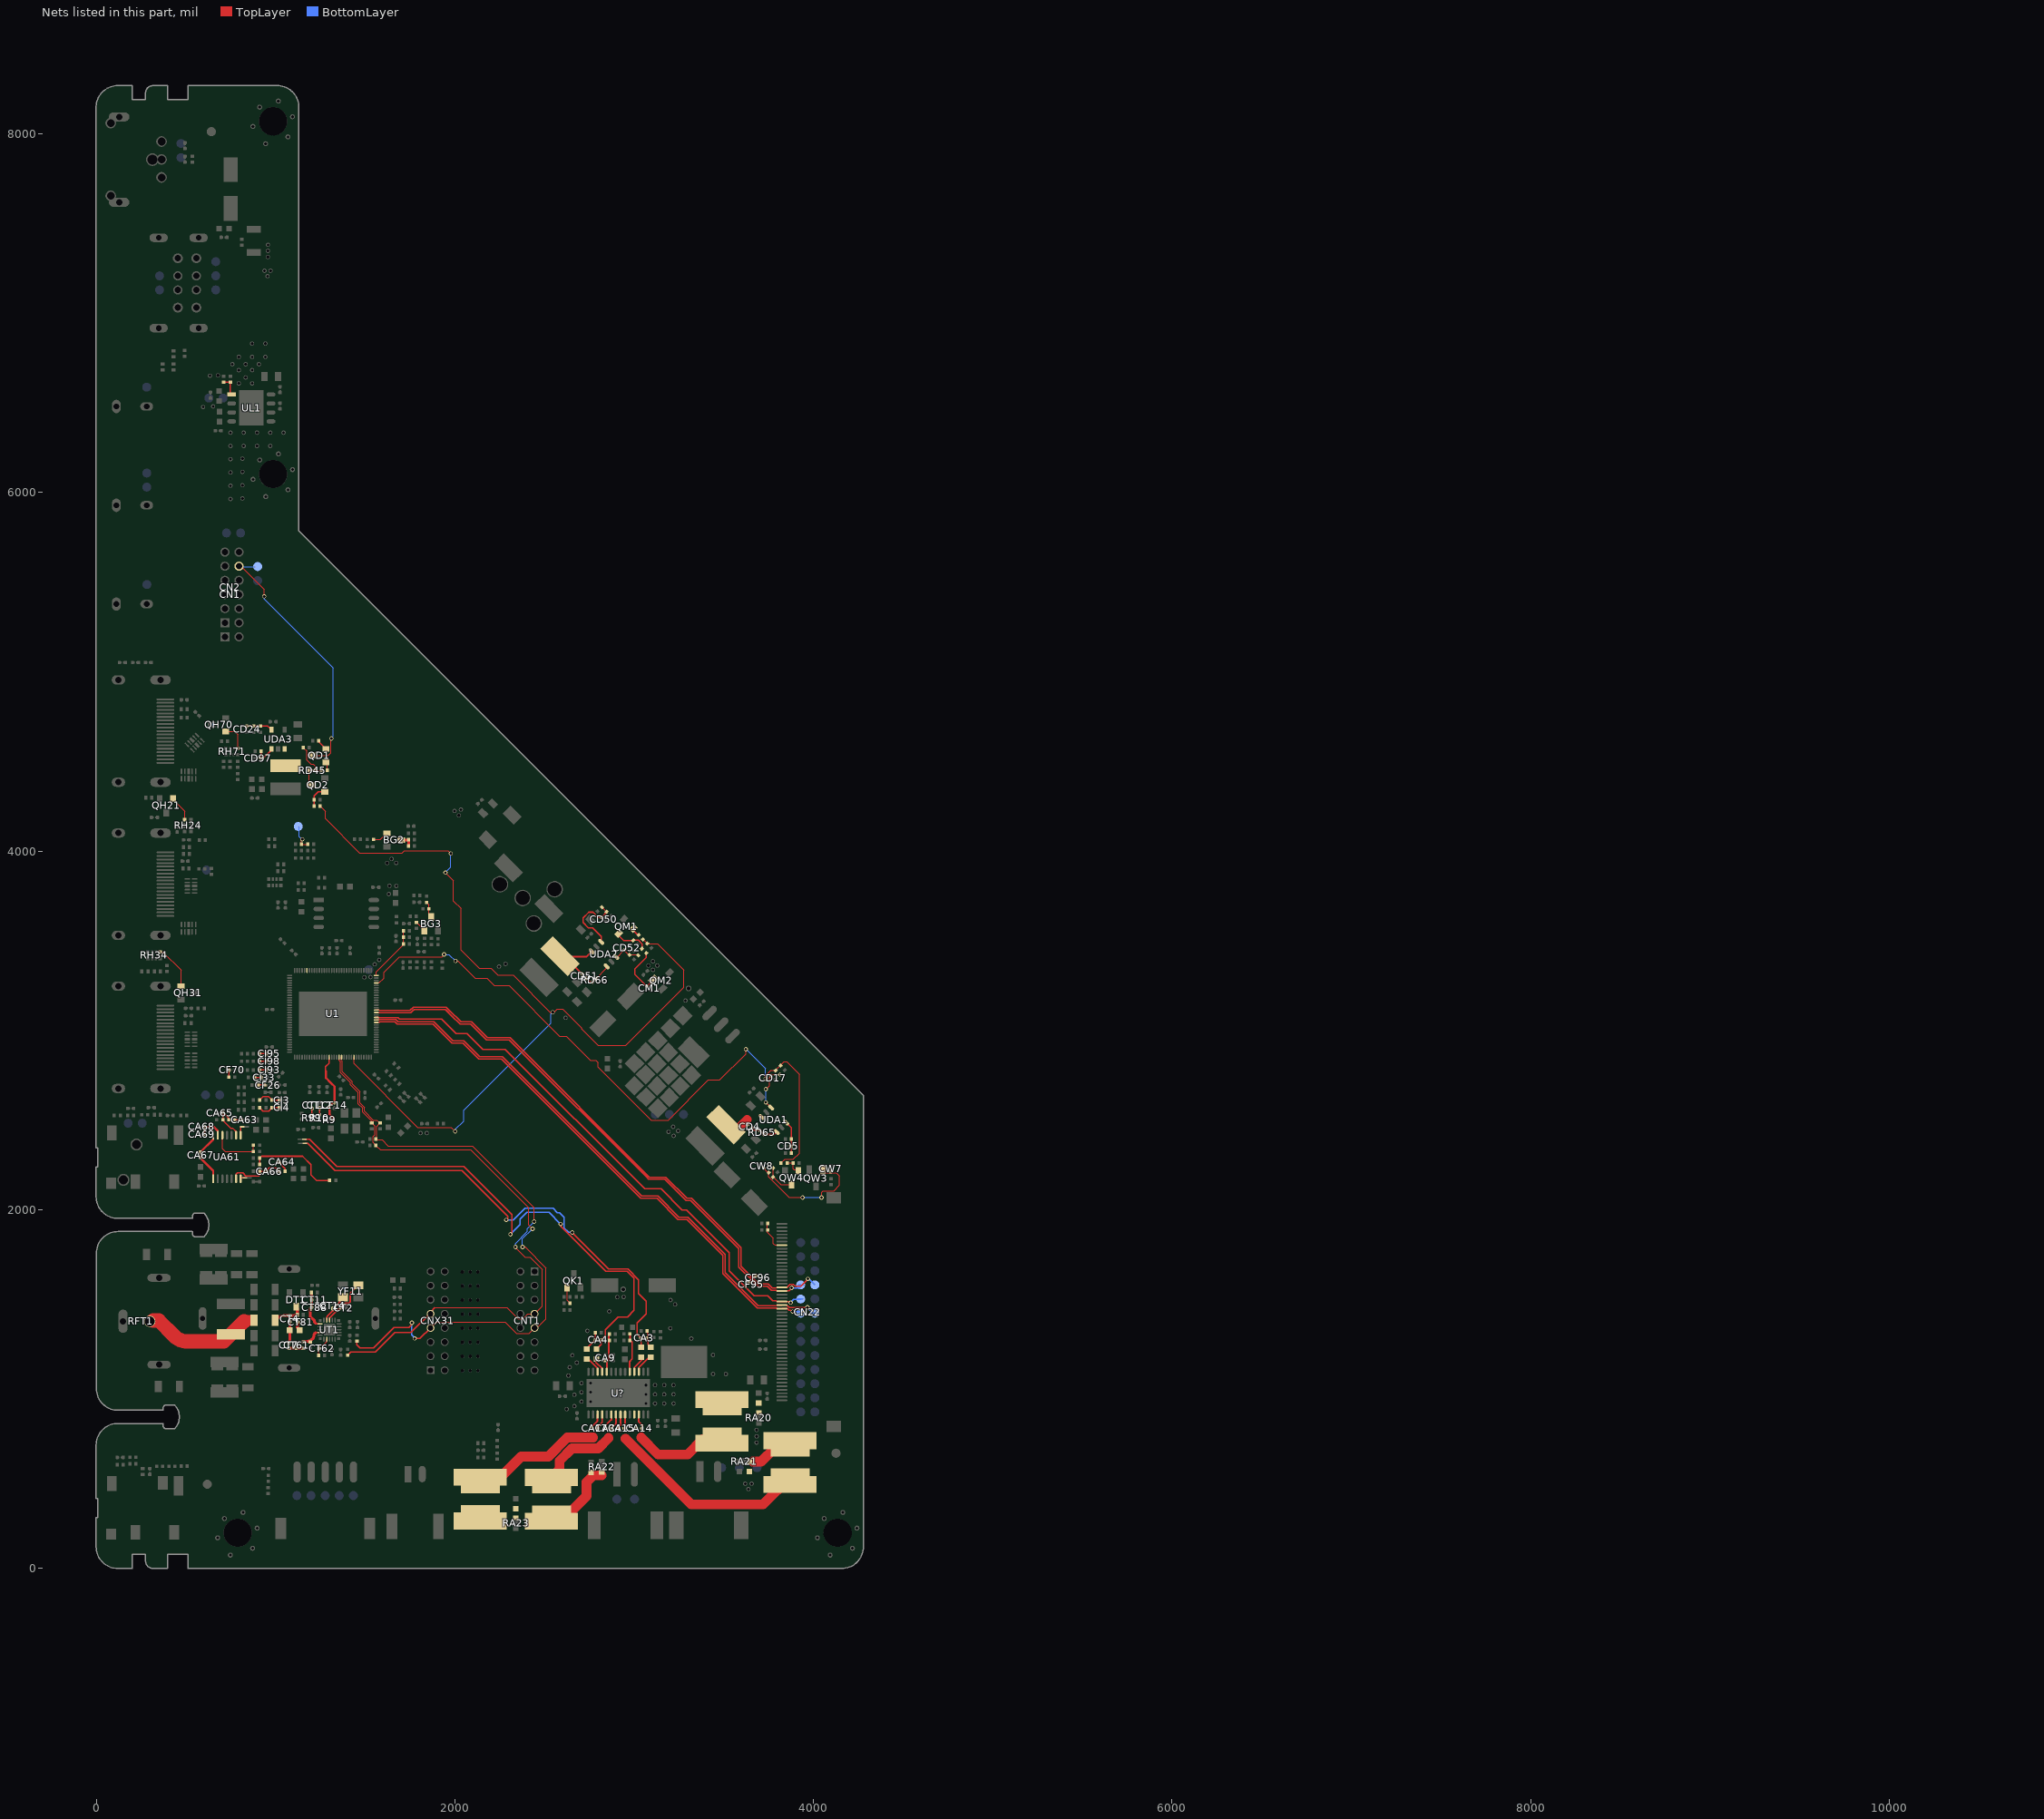
[diagram p0: the nets of this part, all layers, seen from the top]
# Altium PCB MISC105950.PcbDoc (part 12 of 15)
Units mil, origin at the board's own origin, x right, y up, seen from the top; angles counter-clockwise.
Board outline 4280.62 x 8272.76 mil, 2 copper layers (TopLayer, BottomLayer), stack 61.855 mil thick; 541 components, 268 nets, 2324 pads, 1157 vias.

## Via types
v1: diameter 23.62, hole 15.75, TopLayer to BottomLayer, tented both sides, 1087 vias
v2: diameter 23.62, hole 15.75, TopLayer to BottomLayer, 51 vias
v3: diameter 27.56, hole 19.68, TopLayer to BottomLayer, 15 vias
v4: diameter 31.5, hole 19.68, TopLayer to BottomLayer, tented both sides, 4 vias

## Nets (pads, with @x,y where several pads share a name; then routed paths per layer and width w, separated by ;. In a path a pad name is that pad's centre, name@x,y a point inside that pad or via, vN(x,y) a via of type N, cw(c..) or ccw(c..) an arc to the next point about the centre after c; other vN are vias at no path point) (continued)
LVDS_O3P_IC: CN22.29 O3P.1 U1.79 | length 3126.4
  TopLayer w7: U1.79@1560.66,3071.21 1561.61,3072.16 1573.58,3072.16 1574.53,3071.21 1682.5,3071.21 1690.21,3063.5 1924.1,3063.5 2005.42,2982.18 2066.04,2982.18 2154.53,2893.69 2279.87,2893.69 3058.06,2115.5 3148.94,2115.5 3266.39,1998.05 3291.64,1998.05 3529.95,1759.73 3529.95,1657.23 3668.17,1519.01 3744.26,1519.01 3773.37,1489.9 3791.5,1489.9 3794.99,1486.41 CN22.29@3823.43,1486.41 3866.09,1486.41 v1(3872,1480.5)
  BottomLayer w7: v1@3872,1481.5 3888.5,1498 3925.82,1498 O3P.1@3928.5,1500.68 ; O3P.1@3910.18,1500.68 O3P.1@3928.5,1500.68 ; O3P.1@3941.07,1500.68 O3P.1@3928.5,1500.68
LVDS_O4N_IC: CN22.28 O4N.1 U1.78 | length 3165.9
  TopLayer w7: U1.78@1560.66,3057.43 1574.47,3057.43 1576.25,3059.21 1669.47,3059.21 1681.18,3047.5 1882.12,3047.5 1988.44,2941.18 2049.06,2941.18 2137.55,2852.69 2262.89,2852.69 3041.07,2074.5 3131.95,2074.5 3249.41,1957.05 3298.7,1957.05 3505.95,1749.79 3505.95,1647.28 3690.71,1462.53 3790,1462.53 3794.19,1466.72 CN22.28@3823.43,1466.72 ; CN22.28@3851.75,1466.72 3866.24,1452.24 3964.24,1452.24 v1(3966,1454)
  BottomLayer w7: v1(3966,1454) 3966,1450 3994.06,1421.94 O4N.1@4007.24,1421.94 ; O4N.1@4006.68,1421.38 O4N.1@4007.24,1421.94 ; O4N.1@4007.24,1421.3 O4N.1@4007.24,1421.94
LVDS_O4P_IC: CN22.27 O4P.1 U1.77 | length 3079
  TopLayer w7: U1.77@1560.66,3043.65 1561.61,3044.6 1578.61,3044.6 1581.22,3047.21 1664.5,3047.21 1676.21,3035.5 1877.15,3035.5 1983.47,2929.18 2044.09,2929.18 2132.58,2840.69 2257.92,2840.69 3036.1,2062.5 3126.98,2062.5 3244.44,1945.05 3293.73,1945.05 3493.95,1744.82 3493.95,1642.31 3685.74,1450.53 3791.5,1450.53 CN22.27@3794.99,1447.04 ; CN22.27@3823.43,1447.04 3854.46,1447.04 3862.5,1439 v1@3875,1439
  BottomLayer w7: v1(3883,1431) 3919.44,1431 O4P.1@3928.5,1421.94 ; O4P.1@3925.94,1424.5 O4P.1@3928.5,1421.94 ; O4P.1@3941.03,1421.94 O4P.1@3928.5,1421.94
LVDS_OCKN_IC: CF96.2@3676.78,1631.31 CF96.2@3681.65,1626.44 CN22.33 OCKN.1 U1.82 | length 3312.3
  TopLayer w7: U1.82@1560.66,3112.55 1576.22,3112.55 ; 1578,3110.77 1745.38,3110.77 1745.19,3110.96 1748.67,3110.96 ; 1762.22,3124.5 1748.67,3110.96 ; 1955.03,3124.5 1967.93,3111.59 ; 3594.95,1762.61 3594.95,1714 ; CF96.2@3676.49,1631.31 CF96.2@3676.78,1631.31 3663.67,1618.2 3660.9,1618.2 ; v1@3966,1610 3928,1572 3897.72,1572 3886.41,1583.31 3884,1583.31 3869.59,1583.31 3851.42,1565.15 CN22.33@3823.43,1565.15 3794.19,1565.15 3790,1560.95 3770.2,1560.95 3747.15,1584.01 3695.1,1584.01 3660.9,1618.2 ; 1748.67,3110.96 1766.72,3129 1950.53,3129 1967.93,3111.59 ; 1967.93,3111.59 2032.35,3047.18 2092.97,3047.18 2115.07,3025.07 2181.45,2958.69 2306.79,2958.69 3084.98,2180.5 3175.86,2180.5 3293.31,2063.05 3318.56,2063.05 3594.95,1786.65 3594.95,1714 ; 3594.95,1714 3594.95,1684.15 3660.9,1618.2
  BottomLayer w7: v1@3966,1610 3976.66,1610 OCKN.1@4007.24,1579.42
  other v1: 3968,1613
LVDS_OCKP_IC: CF95.2@3639.03,1593.85 CF95.2@3643.9,1588.98 CN22.32 OCKP.1 U1.81 | length 3215.3
  TopLayer w7: U1.81@1560.66,3098.77 1753.45,3098.77 1760.09,3105.41 ; 1767.19,3112.5 1760.09,3105.41 ; 1950.06,3112.5 1981.19,3081.37 ; CF95.2@3639.03,1593.85 3651.63,1606.45 ; v1(3878,1563) 3878,1559 3864.46,1545.46 CN22.32@3823.43,1545.46 3794.99,1545.46 3791.5,1548.95 3765.23,1548.95 3742.18,1572.01 3690.13,1572.01 3582.95,1679.18 3582.95,1781.68 3313.59,2051.05 3288.34,2051.05 3170.89,2168.5 3080.01,2168.5 3070.26,2178.26 2301.82,2946.69 2176.48,2946.69 2087.99,3035.18 2027.38,3035.18 1981.19,3081.37 ; 1760.09,3105.41 1771.69,3117 1945.56,3117 1981.19,3081.37
  BottomLayer w7: v1(3878,1563) 3920.58,1563 OCKP.1@3937,1579.42 ; OCKP.1@3914.42,1579.42 OCKP.1@3928.5,1579.42 OCKP.1@3937,1579.42 ; OCKP.1@3946.58,1579.42 OCKP.1@3937,1579.42
LVDS_SEL: CN22.45 RF4.1 RF5.2 | length 176.6
  TopLayer w5: RF4.1@3741.71,1920.77 3741.71,1873.24 3775.5,1839.45 3775.5,1809.5 3783.63,1801.37 CN22.45@3823.43,1801.37
MAIN_SCL_OUT_IC: CNT1.7 CNX31.9 DK3.K RF43.2 RT2.1 U1.52 | length 3560.2
  TopLayer w5: U1.52@1366.73,2849.72 1366.73,2832.27 1369.84,2829.16 1369.84,2768.82 1425.8,2712.86 1425.8,2701.79 1469.66,2657.93 1469.66,2593.48 1493.5,2569.64 1493.5,2547.85 1542.26,2499.09 1564.05,2499.09 1580.41,2482.73 DK3.K@1581.5,2482.73 1562.83,2464.06 1562.83,2397.36 RF43.2@1558.96,2393.5 1564.15,2388.31 1594,2388.31 1627.31,2355 2095.83,2355 2441,2009.83 2441,1961.5 ; 1888,1452 2289.13,1452 2352.4,1388.74 2376.55,1388.74 2405.7,1417.89 CNT1.7@2443.21,1417.89 2485.5,1460.18 2485.5,1665.73 2417.05,1734.19 2390,1734.19 v1@2336.5,1787.69 ; v1@2441,1931.5 2441,1961.5 ; v1(2441,1932.5) 2441,1961.5
  TopLayer w7: RT2.1@1401,1187.77 1417.73,1204.5 1555.94,1204.5 1664.44,1313 1753.89,1313 1858.84,1417.95 CNX31.9@1863.21,1417.95 1863.21,1427.21 1888,1452
  BottomLayer w5: v1(2336.5,1791) 2336.5,1810.64 2403,1877.14 2403,1893.5 v1@2441,1931.5
MAIN_SDA_IO_IC: CNT1.9 CNX31.7 DK2.K RF44.2 RT3.1 U1.51 | length 3623.1
  TopLayer w5: U1.51@1351.85,2848.62 U1.51@1352.95,2849.72 1352.95,2831.91 1359.84,2825.02 1359.84,2764.68 1416.7,2707.82 1416.7,2696.75 1459.66,2653.79 1459.66,2589.34 1483.5,2565.5 1483.5,2543.71 1534.5,2492.71 DK2.K@1534.5,2482.73 1552.83,2464.41 1552.83,2416.67 1542.61,2406.45 1542.61,2373.86 RF44.2@1558.96,2357.5 1582.46,2334 2087.13,2334 2410.5,2010.63 2410.5,1913.96 v1@2431.96,1892.5 ; CNX31.7@1863.21,1339.21 1897,1373 2280,1373 2343,1310 2414.06,1310 CNT1.9@2443.21,1339.15 2455.15,1339.15 2506.5,1390.5 2506.5,1674.43 2389.93,1791 v1(2376.5,1791)
  TopLayer w7: RT3.1@1452,1265.27 1452,1245 1468.5,1228.5 1546,1228.5 1658,1340.5 1742.5,1340.5 1758.81,1356.81 v1(1758.81,1368.56) ; v1(1775,1280.5) 1804.5,1280.5 CNX31.7@1863.21,1339.21
  BottomLayer w5: v1(2376.5,1791) 2376.5,1836.5 v1(2432.5,1892.5)
  BottomLayer w7: v1@1761.31,1366.06 v1(1758.81,1368.56) 1758.81,1299.95 1775,1283.77 v1(1775,1280.5)
MHL_5V_IN_IC: U1.123
NetBG2_B: BG2.B RG1.1 | length 83.8
  TopLayer w5: RG1.1@1544.23,4064.5 1583.5,4064.5 BG2.B@1615,4096
NetBG2_C: BG2.C RG6.2 RG66.1 | length 84.6
  TopLayer w5: BG2.C@1693.03,4058 BG2.C@1698.53,4058
  TopLayer w15: BG2.C@1698.53,4061 1738.02,4061 1740.77,4063.75 RG66.1@1740.77,4028
NetBG3_B: BG3.B RG2.1 | length 64.1
  TopLayer w5: RG2.1@1784.5,3601.73 1826.5,3559.73 BG3.B@1826.5,3555
NetBG3_C: BG3.C RG7.2 RG67.1 | length 91.5
  TopLayer w5: RG7.2@1841,3713.77 1854.73,3700.04 RG67.1@1854.73,3677.5 1854.73,3645.3 BG3.C@1867,3633.03
NetCA3_1: CA3.1 CA6.1 RA4.JP_1K | length 2721.9
  TopLayer w7: RA4.JP_1K@1162,2368.34 1179.08,2368.34 1330.42,2217 2038.66,2217 2293.5,1962.16 v1@2293.5,1942 ; v1@2653,1871.5 2856,1668.5 2963.78,1668.5 3024,1608.28 3024,1530.59 3066.95,1487.63 3066.95,1417.74 3015.13,1365.91 3015.13,1303.64 CA3.1@3036.27,1282.5 3038,1280.77 CA6.1@3038,1231.81 ; CA6.1@3041.77,1226.04 CA6.1@3041.77,1231.81
  BottomLayer w7: v1@2285,1938.51 v1(2285,1942) 2324.82,1942 2390.13,2007.31 2546.16,2007.31 2570.97,1982.5 2584,1982.5 2609.31,1957.19 2609.31,1907 2609.31,1895.94 2633.25,1872 v1(2653.5,1872)
NetCA3_2: CA3.2@3062.85,1282.5 CA3.2@3069.74,1282.5 CA5.1 RA3.2 | length 102.4
  TopLayer w7: 3072.5,1310.5 3072.5,1272.73 3075.23,1270 3075.23,1247.08 CA5.1@3102,1220.31
NetCA4_1: CA4.1 CA11.1 RA14.2 | length 107.6
  TopLayer w7: CA11.1@2739.5,1222.31 2739.5,1230.44 CA4.1@2782.3,1273.23 RA14.2@2782.29,1312.23
NetCA4_2: CA4.2@2808.87,1273.23 CA4.2@2815.76,1273.23 CA10.1 RA5.JP_1K | length 2861.6
  TopLayer w7: RA5.JP_1K@1160,2392.34 1189.02,2392.34 1340.37,2241 2048.61,2241 2317.5,1972.11 2317.5,1870.5 v1(2309,1862) ; 2589,1907.3 2839.8,1656.5 2958.81,1656.5 2998,1617.31 2998,1437 2961.5,1400.5 2908.5,1400.5 2837.5,1329.5 2837.5,1294.97 CA4.2@2815.76,1273.23 2815.76,1248.14 CA10.1@2788.94,1221.32
  BottomLayer w7: v1(2309,1862) 2363,1916 2363,1946.24 2400.07,1983.31 2524.47,1983.31 v1@2588.28,1919.5
  other v1: 2589,1919.5
NetCA5_2: CA5.2 U?.3 | length 114.2
  TopLayer w7: U?.3@3025.36,1094.5 3025.36,1117.86 3083.69,1176.19 CA5.2@3092,1176.19
NetCA6_2: CA6.2 U?.4 | length 164.3
  TopLayer w7: U?.4@2999.77,1094.5 2999.77,1118.77 ; CA6.2@3038,1176.19 3038,1157 2999.77,1118.77 ; CA6.2@3047.5,1164.69 3045.69,1164.69 2999.77,1118.77
NetCA9_2: CA9.2@2837.44,1155.77 CA9.2@2837.44,1162.66 RA10.2 RA11.2 U?.10 | length 219.3
  TopLayer w10: CA9.2@2837.44,1155.77 2847.7,1155.77 2858.07,1166.13 2858.07,1303.37 RA11.2@2860.21,1305.5 ; U?.10@2846.23,1094.5 2846.23,1146.98 ; RA10.2@2858.07,1262.37 RA10.2@2859.21,1263.5
NetCA10_2: CA10.2 U?.11 | length 86.3
  TopLayer w7: CA10.2@2786.5,1166.69 2786.5,1147.5 2820.64,1113.36 U?.11@2820.64,1094.5
NetCA11_2: CA11.2 U?.12 | length 93.8
  TopLayer w7: CA11.2@2742.98,1166.69 2795.05,1114.62 U?.12@2795.05,1094.5
NetCA14_1: CA14.1 U?.26 | length 76.9
  TopLayer w10: U?.26@3025.36,854.34 3025.36,825.78 3025.5,825.64 3025.5,815.23 3043.73,797 CA14.1@3043.73,785
NetCA14_2: CA14.2@3010.26,779 CA14.2@3017.15,779 LA1.2 LA5.S U?.25 | length 417.8
  TopLayer w55: 3038,727.5 3132.33,633.17 3297.55,633.17 LA1.2@3381.83,717.45
NetCA15_1: CA15.1 U?.22 | length 79.8
  TopLayer w10: CA15.1@2912.27,779 2912.27,786.68 2923,797.41 U?.22@2923,854.34
NetCA15_2: CA15.2@2938.85,779 CA15.2@2945.74,779 LA2.F LA3.1 U?.23 | length 1208.6
  TopLayer w10: CA15.2@2945.74,779 2948.59,781.85 U?.23@2948.59,854.34
  TopLayer w55: 2951.25,721.75 3318,355 3718.37,355 LA2.F@3869,505.63
NetCA17_1: CA17.1 U?.17 | length 88.1
  TopLayer w10: CA17.1@2764.27,779 2764.27,789.32 2795.05,820.09 U?.17@2795.05,854.34
NetCA17_2: CA17.2@2790.85,779 CA17.2@2797.74,779 LA4.F LA8.1 U?.18 | length 845.4
  TopLayer w10: CA17.2@2797.74,779 2797.74,789.74 2820.64,812.64 U?.18@2820.64,854.34
  TopLayer w55: LA4.F@2140.5,466.87 LA8.1@2140.5,506.05 2253.05,506.05 2369.32,622.32 2520.86,622.32 2625.79,727.25 2770.25,727.25
NetCA20_2: CA20.2 LA1.1 LA5.F RA20.1
NetCA21_1: CA21.1 LA2.S LA3.2 RA21.1 | length 239.9
  TopLayer w55: 3661.14,594 3708.5,594 3785.87,671.37 LA2.S@3869,671.37
NetCA22_2: CA22.2 LA6.2 LA7.S RA22.1 | length 415.2
  TopLayer w55: LA7.S@2538,300.17 2632.67,300.17 2733.5,401 2733.5,479 2770.86,516.36 2818,516.36
NetCA23_1: CA23.1 LA4.S LA8.2 RA23.1
NetCA34_1: CA34.1 U?.21 | length 85.8
  TopLayer w10: CA34.1@2872.23,779 2897.41,804.18 U?.21@2897.41,854.34
NetCA34_2: CA34.2@2838.76,779 CA34.2@2845.65,779 LA6.1 LA7.F U?.20 | length 527.5
  TopLayer w10: CA34.2@2838.76,779 2838.76,794.76 2871.82,827.82 U?.20@2871.82,854.34
  TopLayer w55: LA6.1@2538,505.09 2583,550.09 2583,597.5 2652.75,667.25 2799.21,667.25 2856,724.04 2856,726
NetCA63_2: CA63.2@808.03,2501 CA63.2@814.92,2501 RA62.1 | length 36.3
  TopLayer w7: RA62.1@771.73,2501 CA63.2@808.03,2501
NetCA64_2: CA64.2@1018.27,2266 CA64.2@1025.16,2266 RA63.1 | length 62.1
  TopLayer w7: CA64.2@1018.27,2261.69 1051.73,2228.23 RA63.1@1051.73,2213.5
NetCA65_1: CA65.1 RA62.2 RA66.1 UA61.2 | length 221.3
  TopLayer w8: CA65.1@711,2544 CA65.1@707.09,2540.09 ; RA62.2@738.27,2501 738.27,2508.91 CA65.1@707.09,2540.09 ; UA61.2@778.36,2414.61 778.36,2435.14 761.5,2452 750.5,2452 704.23,2498.27 RA66.1@704.23,2501 704.23,2537.23 CA65.1@707.09,2540.09
NetCA66_2: CA66.2@946,2213.5 CA66.2@952.89,2213.5 RA63.2 RA67.1 UA61.13 | length 312.6
  TopLayer w7: UA61.13@778.36,2171.5 778.36,2195.86 786.61,2204.11 815.89,2204.11 832,2188 905,2188 909.23,2192.23 RA67.1@909.23,2213.5 CA66.2@946,2213.5 964.34,2231.84 999.92,2231.84 RA63.2@1018.26,2213.5
NetCA67_1: CA67.1 UA61.8 | length 144.9
  TopLayer w12: CA67.1@580,2287.27 650.41,2216.86 UA61.8@650.41,2171.5
NetCA67_2: CA67.2@580,2313.84 CA67.2@580,2320.73 UA61.7 | length 123
  TopLayer w12: CA67.2@580,2320.73 650.41,2391.14 UA61.7@650.41,2414.61
NetCA68_1: CA68.1 CA69.1 UA61.6 | length 148.8
  TopLayer w12: CA69.1@602.39,2420 CA68.1@602.39,2461.69 652.81,2461.69 676,2438.5 UA61.6@676,2414.61
NetCD4_1: CD4.1 LD1.1 UDA1.6 | length 164.7
  TopLayer w50: LD1.1@3512.01,2473.01 3555.51,2429.51 3628.5,2502.5
NetCD4_2: CD4.2@3650.5,2457 CD4.2@3655.37,2452.13 RD65.1 | length 47.8
  TopLayer w8: CD4.2@3655.37,2452.13 3664.79,2442.71 RD65.1@3699.29,2442.71
NetCD5_1: CD5.1 RD31.1 RD35.2 UDA1.3 | length 183.4
  TopLayer w8: UDA1.3@3846.71,2485.19 3876,2455.89 RD35.2@3876,2393 3876,2316.11 RD31.1@3877.57,2314.54
NetCD17_1: CD17.1 RD1.2 UDA1.4 | length 254.7
  TopLayer w5: v1@3733.5,2597.5 3752.5,2578.5 UDA1.4@3752.5,2568.71 ; v1(3733.5,2671.5) 3753.5,2691.5 3753.5,2737 3762.25,2745.75 3769.5,2753 RD1.2@3812.5,2753 ; RD1.2@3807.18,2752.68 RD1.2@3812.31,2752.68
  BottomLayer w5: v1@3733.5,2598.02 v1(3733.5,2671.5)
  other v1: 3733.5,2597.5
NetCD24_1: CD24.1 RD81.1 RD88.2 UDA3.5 | length 138.8
  TopLayer w8: CD24.1@844.24,4696.73 956.01,4696.73 UDA3.5@975.1,4677.63
NetCD50_1: CD50.1 RD52.2 RD53.1 UDA2.4 | length 397.4
  TopLayer w8: UDA2.4@2815.19,3492.7 2815.19,3523.81 2767.5,3571.5 2744,3571.5 2714,3601.5 2714,3627.03 2745.47,3658.5 2769.5,3658.5 2797.17,3630.83 CD50.1@2817.17,3630.83 2845.67,3659.32 RD53.1@2845.67,3661.33 2844.33,3661.33 RD52.2@2818.83,3686.83
NetCD51_1: CD51.1 LD11.1 UDA2.6 | length 341.5
  TopLayer w10: LD11.1@2585.6,3412.6 2587.89,3410.31 2732.79,3410.31 UDA2.6@2762.29,3439.81 ; LD11.1@2602.1,3420.1 2708.37,3313.83 CD51.1@2709.67,3313.83
NetCD51_2: CD51.2@2728.46,3295.04 CD51.2@2733.33,3290.17 RD66.1 | length 62.3
  TopLayer w6: 2747.5,3276 CD51.2@2733.33,3290.17 2756.5,3267 RD66.1@2766,3267
NetCD52_1: CD52.1 RD54.2 RD91.1 UDA2.3 | length 153.8
  TopLayer w6: UDA2.3@2901,3405.5 CD52.1@2944.5,3449 ; CD52.1@2944.89,3448.27 2944.89,3444.61 RD91.1@2970.5,3419 ; CD52.1@2952.39,3450.27 CD52.1@2952.88,3450.27 ; RD91.1@2972.89,3420.77 3018.73,3420.77 RD54.2@3023,3416.5
NetCD97_1: CD97.1 RD2.2 UDA3.1 | length 121.7
  TopLayer w8: RD2.2@917,4556.5 917,4518 CD97.1@917.5,4517.5 929,4517.5 975.1,4563.6 UDA3.1@975.1,4569.37
NetCF14_2: CF14.2@1326.5,2590.58 CF14.2@1326.5,2597.47 R9.1 U1.47 | length 467.9
  TopLayer w8: 1277.04,2736.38 1277.04,2796.34 1297.83,2817.14 U1.47@1297.83,2849.72
  TopLayer w12: 1280.04,2772.69 1280.04,2733.38 1309.21,2704.21 ; 1293.31,2720.1 1309.21,2704.21 ; 1299.84,2567 1299.84,2578.3 ; R9.1@1319.27,2500.5 1319.27,2511.06 1312.82,2517.5 1312.5,2517.5 1299.84,2530.16 1299.84,2578.3 ; 1299.84,2578.3 1328.31,2606.77 1328.31,2685.1 1309.21,2704.21
NetCF26_2: CF26.2@939.26,2693.5 CF26.2@946.15,2693.5 RF12.1 | length 37.3
  TopLayer w7: RF12.1@908.73,2694.5 CF26.2@946,2694.5
NetCF70_2: CF70.2@738.26,2778 CF70.2@745.15,2778 RF19.1 | length 39.5
  TopLayer w7: RF19.1@738.27,2739.5 CF70.2@738.27,2779
NetCI3_2: CI3.2@1018.26,2610 CI3.2@1025.15,2610 RI13.1 RI14.1 | length 124.6
  TopLayer w8: RI13.1@909.23,2610 928.07,2628.84 960.63,2628.84 RI14.1@979.47,2610 CI3.2@1018.26,2610
NetCI4_2: CI4.2@1018.26,2568 CI4.2@1025.15,2568 RI15.1 RI16.1 | length 124.2
  TopLayer w7: RI15.1@909.23,2568 927.57,2549.66 961.13,2549.66 RI16.1@979.47,2568 CI4.2@1018.26,2568
NetCI33_1: CI33.1 RI22.2 | length 37.5
  TopLayer w7: RI22.2@881.23,2736.5 CI33.1@918.77,2736.5
NetCI93_1: CI93.1 RI26.2 | length 38
  TopLayer w7: RI26.2@908.73,2778.5 CI93.1@946.77,2778.5
NetCI95_1: CI95.1 RI24.2 | length 38
  TopLayer w7: RI24.2@908.73,2869 CI95.1@946.77,2869
NetCI98_1: CI98.1 RI38.2 | length 38
  TopLayer w7: RI38.2@908.73,2827.5 CI98.1@946.77,2827.5
NetCM1_1: CM1.1 QM2.G RM4.2 | length 303.9
  TopLayer w8: RM4.2@3066.33,3431.17 3066.33,3405.83 3002,3341.5 3002,3312.5 3069.67,3244.83 CM1.1@3072.54,3247.7 ; CM1.1@3072.54,3245.46 CM1.1@3072.54,3247.7 ; CM1.1@3072.54,3250.33 CM1.1@3072.54,3247.7 ; QM2.G@3098.15,3291.04 3098.15,3273.3 CM1.1@3072.54,3247.7
NetCT1_2: CT1.2@1201.5,2565 CT1.2@1201.5,2571.89 R99.1 | length 36.5
  TopLayer w7: R99.1@1201.5,2528.5 CT1.2@1201.5,2565
NetCT2_2: CT2.2@1360.26,1451 CT2.2@1367.15,1451 UT1.16 YF11.1 | length 279.3
  TopLayer w7: UT1.16@1299.5,1383.15 1299.5,1394.83 1354.67,1450 CT2.2@1359.76,1450
  TopLayer w10: CT2.2@1359.76,1450 1386.26,1476.5 1407,1476.5 1414,1483.5 1414,1531.03 1459.94,1576.96 YF11.1@1460.31,1576.96 ; YF11.1@1467.81,1574.46 YF11.1@1470.31,1576.96
NetCT4_1: CT4.1 CT7.2@1072.5,1252.35 CT7.2@1072.5,1259.24 LT80.1 | length 115.9
  TopLayer w15.8: CT7.2@1072.5,1259.24 ccw(c1060.43,1271.31) 1077.5,1271.31 CT4.1@1077.5,1373.77
NetCT4_2: CT4.2@1077.5,1400.35 CT4.2@1077.5,1407.24 CT40.2 DT1.2 LT2.2 | length 181.9
  TopLayer w15.8: CT40.2@996.09,1379.62 1010.51,1394.04 cw(c1043,1361.56) 1043,1407.5 1092.65,1407.5 ccw(c1092.65,1443.35) 1117.97,1417.97 LT2.2@1116.5,1416.5 ; DT1.2@1116,1457.47 cw(c1106.91,1448.38) 1119.76,1448.38 LT2.2@1119.76,1413
NetCT7_1: CT7.1 CT61.1 LT3.1 | length 82.1
  TopLayer w15.8: CT7.1@1072.5,1225.77 CT61.1@1114.5,1225.77 1153.29,1225.77 ccw(c1153.29,1227.48) LT3.1@1154.5,1226.27
NetCT11_2: CT11.2@1198.25,1496.4 CT11.2@1205.14,1496.4 CT88.1 FT2.1 UT1.20 | length 200.2
  TopLayer w7: 1221,1366 1225.5,1361.5 UT1.20@1246.35,1361.5
  TopLayer w15.8: 1199.27,1523.5 1199.27,1483.5 1199.27,1454.91 1191.5,1447.14 1191.5,1404 1215.5,1380 1215.5,1371.5 1221,1366
NetCT12_2: CT12.2@1244,2565 CT12.2@1244,2571.89 R10.1 | length 36.5
  TopLayer w7: R10.1@1244,2528.5 CT12.2@1244,2565
NetCT14_2: CT14.2@1318,1446.26 CT14.2@1318,1453.15 UT1.17 YF11.3 | length 171.2
  TopLayer w7: UT1.17@1283.75,1396.06 UT1.17@1283.75,1383.15 1283.75,1400.89 1290.29,1407.43
  TopLayer w10: 1290.29,1407.43 1318,1435.14 ; CT14.2@1318,1446.26 1319.92,1446.26 YF11.3@1383.69,1510.04
NetCT62_1: CT62.1 RT1.2 UT1.3 | length 121.1
  TopLayer w5: RT1.2@1238.77,1185.5 1239.77,1186.5 CT62.1@1239.77,1224.5 1239.77,1238.27 1246.5,1245 1265.54,1245 1283.75,1263.21 UT1.3@1283.75,1276.85
NetCT81_1: CT81.1 LT80.2 | length 51.4
  TopLayer w15.8: CT81.1@1120.27,1373 1120.27,1340.04 LT80.2@1133.31,1327
NetCW7_1: CW7.1 CW8.2@3717.72,2235.01 CW8.2@3722.59,2230.14 QW3.G RW12.2 | length 706.5
  TopLayer w5: CW8.2@3722.59,2230.14 3747.42,2205.3 RW12.2@3749.92,2205.3 3749.92,2180.78 3863.7,2067 v1(3938.5,2067) ; v1(4044.5,2067) 4044.5,2096.15 4052.49,2104.14 4113.64,2104.14 4144.59,2135.09 4144.59,2187.72 4127.66,2204.66 4095.5,2204.66 QW3.G@4047,2204.66
  BottomLayer w5: v1(3938.5,2067) v1(4044.5,2067)
NetLD21_2: LD21.2 UDA3.3
NetLT3_2: LT3.2 LT4.2 UT1.23 | length 120.6
  TopLayer w7: 1221.7,1311.2 1224.75,1314.25 UT1.23@1246.35,1314.25
  TopLayer w15.8: LT3.2@1154,1263.74 1168.65,1263.74 ccw(c1168.65,1315.85) 1205.5,1279 ccw(c1191.01,1293.49) 1211.5,1293.49 cw(c1233.26,1293.49) 1222.59,1312.45
NetQD1_B: QD1.B RD44.1 | length 47.9
  TopLayer w5: QD1.B@1279.8,4494.5 1288.03,4486.27 RD44.1@1288.03,4450
NetQD1_E: QD1.E RD42.1 | length 62.5
  TopLayer w8: RD42.1@1238.73,4615 1238.73,4610.57 QD1.E@1279.8,4569.5
NetQD2_B: QD2.B RD46.2 RD47.1 | length 126.2
  TopLayer w7: RD46.2@1213.77,4251 1213.77,4308.77 1236,4331 QD2.B@1273,4331
NetQD2_C: QD2.C RD45.1 | length 72.9
  TopLayer w5: QD2.C@1186.83,4377.13 RD45.1@1186.83,4450
NetQH21_B: QH21.B RH24.8 | length 143.6
  TopLayer w5: QH21.B@426.5,4292.5 426.5,4286.5 491.5,4221.5 RH24.8@491.5,4175.81
NetQH31_B: QH31.B RH34.1 | length 248
  TopLayer w5: RH34.1@354,3436.5 369.5,3436.5 471,3335 QH31.B@471,3246
NetQH70_B: QH70.B RH71.8 | length 152.4
  TopLayer w5: QH70.B@720,4667 721.42,4667 769,4667 787.81,4648.19 RH71.8@787.81,4573.5 RH71.8@786.31,4575
NetQK1_B: QK1.B RK15.2 | length 90.3
  TopLayer w5: QK1.B@2624.87,1560 2624.87,1494.13 2641.23,1477.77 RK15.2@2641.23,1476.5
NetQM1_B: QM1.B RM2.2 | length 46.8
  TopLayer w8: QM1.B@2990.3,3561.27 3020.24,3531.33 RM2.2@3024.67,3531.33
NetQM1_C: QM1.C RM3.1 RM4.1 | length 184.6
  TopLayer w8: QM1.C@2908.25,3532.96 2940.38,3500.83 2993.67,3500.83 RM3.1@2995.17,3502.33 ; RM3.1@2994.67,3502.33 RM3.1@2995.17,3502.33 ; RM4.1@3042.67,3454.83 3042.67,3482.33 3022.67,3502.33 RM3.1@2995.17,3502.33
NetQW4_B: QW4.B RW13.2 RW14.1 | length 98
  TopLayer w5: RW13.2@3852,2259.5 RW14.1@3886.04,2259.5 3886.04,2227.46 3892,2221.5 QW4.B@3915.5,2221.5
NetQW4_C: QW4.C RW10.1 RW12.1 | length 180.1
  TopLayer w5: RW10.1@3774.67,2231.33 3774.67,2182.72 RW12.1@3773.59,2181.64 3817.26,2137.97 QW4.C@3885.5,2137.97
NetRA8_2: RA8.2 RA9.2 U?.5 | length 224.1
  TopLayer w10: U?.5@2974.18,1094.5 2974.18,1152.75 2987.75,1166.32 2987.75,1260.75 2975.73,1272.77 RA8.2@2975.73,1308
NetRA64_JP_1K: RA64.JP_1K UA61.1 | length 55.2
  TopLayer w7: UA61.1@803.95,2414.61 803.95,2460.95 804.54,2461.54 RA64.JP_1K@812.56,2461.54
NetRA65_JP_1K: RA65.JP_1K UA61.14 | length 19.9
  TopLayer w7: UA61.14@808.45,2176 RA65.JP_1K@828.4,2176
NetRA68_2: RA68.2 RA69.2 UA61.5 | length 291.4
  TopLayer w5: UA61.5@701.59,2414.61 701.59,2339.41 717.25,2323.75 RA68.2@875.77,2323.75 RA69.2@875.77,2359.25
NetRA70_1: RA70.1 RA71.2 RA72.1 | length 525
  TopLayer w7: RA71.2@909.23,2251.5 909.23,2285 RA72.1@909.23,2287.5
  TopLayer w8: RA72.1@909.23,2285 RA72.1@910.48,2286.25 ; RA72.1@909.23,2287.5 RA72.1@910.48,2286.25 ; RA72.1@911.73,2285 RA72.1@910.48,2286.25 ; RA70.1@1300.77,2162.5 1226.9,2162.5 1195.61,2193.8 1195.61,2250.7 1149.46,2296.84 921.08,2296.84 RA72.1@910.48,2286.25
NetRD43_1: RD43.1 RD44.2 RD45.2 RD45.3 | length 196.6
  TopLayer w5: RD43.1@1153.54,4576.5 1172.15,4557.89 1172.15,4507.35 1195.5,4484 1209.5,4484 1220.3,4473.2 RD45.2@1220.3,4450 RD44.2@1254.57,4450
NetRD65_2: RD65.2 RD65.3 UDA1.1 | length 76.1
  TopLayer w8: RD65.2@3723.33,2418.67 3780.19,2418.67 UDA1.1@3793.81,2432.29
NetRD66_2: RD66.2 RD66.3 UDA2.1 | length 87.8
  TopLayer w6: RD66.2@2789.83,3291.33 2844.5,3346 UDA2.1@2844.5,3356.5
NetRH102_2: RH102.2 RH105.1 RXD.1 | length 145.3
  TopLayer w5: v1(1147.64,4065.41) 1143.16,4060.93 RH102.2@1143.16,4037.75 RH105.1@1177.2,4037.75
  BottomLayer w5: RXD.1@1125,4137.5 1131.31,4131.19 1131.31,4081.19 1147.09,4065.41 v1(1147.64,4065.41)
NetRL31_1: RL31.1 RL32.2 UL1.1 | length 113.9
  TopLayer w8: RL31.1@709.5,6615.27 747.5,6615.27 RL32.2@747.5,6620.27 ; UL1.1@746.5,6554.45 RL32.2@746.5,6615.27 ; UL1.1@747.5,6554.45 747.5,6553.45 UL1.1@753.95,6547
PANEL_EN_OUT_IC: RD1.1 RD28.2 RW13.1 U1.93 | length 3806.6
  TopLayer w5: U1.93@1560.66,3264.12 1576.61,3264.12 1603.94,3291.45 1603.94,3324.44 1690,3410.5 1735,3410.5 ; 1704,3410.5 1735,3410.5 ; 1741.5,3410.5 1735,3410.5 ; v1(1939,3423) 1926.5,3410.5 1735,3410.5 ; v1(2002.5,3386.5) 2016.37,3386.5 2112.37,3290.5 2178,3290.5 2219.31,3249.19 2300.62,3249.19 2582.81,2967 2621.25,2967 2755.87,2832.39 2785.11,2832.39 2797.5,2820 2797.5,2795.44 3093.94,2499 3189.02,2499 3413.52,2723.5 3477.09,2723.5 3622.5,2868.91 v1(3622.5,2894.5) ; v1@3731.5,2729 3731.5,2745 3762.85,2776.35 RD1.1@3788.65,2776.35 3836.4,2824.09 3851.59,2824.09 3920.6,2755.08 3920.6,2314.71 3886.39,2280.5 3839.54,2280.5 RW13.1@3818.54,2259.5
  BottomLayer w5: v1(1939,3423) 1966,3423 v1(2002.5,3386.5) ; v1(3622.5,2894.5) 3731,2786 v1(3731,2729) ; v1@3729.5,2726 v1@3729.5,2730
POWER_EN_OUT_IC: RD46.1 RM1.1 RM2.1 U1.57 | length 5177.5
  TopLayer w5: RD46.1@1247.23,4251 1277,4221.23 1277,4180 1467.5,3989.5 1705,3989.5 1716,4000.5 1960,4000.5 v1@1974,3986.5 ; U1.57@1435.63,2849.72 1435.63,2813.34 1789.97,2459 1978,2459 v1(2000.5,2436.5) ; v1(1946,3879.5) 1991.5,3834 1991.5,3721.07 2033.31,3679.25 2033.31,3447.34 2135.15,3345.5 2200.78,3345.5 2238.47,3307.81 2323.69,3307.81 2533,3098.5 2548.5,3098.5 2569,3119 ; v1@2554,3104 2569,3119 ; RM2.1@3044.83,3511.17 3044.83,3510.17 RM1.1@3068.17,3486.83 ; RM1.1@3071.67,3483.33 3129.17,3483.33 3276.5,3336 3276.5,3239.32 2952.57,2915.39 2798.43,2915.39 2707.39,3006.43 2707.39,3011.81 2600.19,3119 2569,3119
  BottomLayer w5: v1(1946,3879.5) 1976,3909.5 v1(1976,3986.5) ; v1@2000.5,2446.5 2048.17,2494.17 2048.17,2553.5 2534.91,3040.24 ; 2534.91,3087.91 2534.91,3040.24 ; v1(2545,3100.5) 2545,3099.5 2534.91,3089.41 2534.91,3040.24
PW_ON: CN1.12 CN2.10 PWON.1 QD1.C | length 1517.2
  TopLayer w5: CN2.10@794.34,5588.8 805.2,5588.8 934.67,5459.33 v1@934.67,5420.83 ; QD1.C@1201.77,4532.5 1241,4532.5 ; 1281.5,4532.5 1241,4532.5 ; v1(1310,4628) 1306.98,4631.02 1306.98,4547.48 1292,4532.5 1241,4532.5
  TopLayer w8: v1@934.67,5420.83 v1(935,5420.5)
  BottomLayer w5: CN2.10@797.27,5585.88 PWON.1@885.45,5585.88 ; v1(935,5420.5) 935,5406.82 1320.28,5021.54 1320.28,4638.28 v1(1310,4628)
PWM1: DI3.K RF13.1 RG3.2 U1.96 | length 312.8
  TopLayer w5: U1.96@1560.66,3305.46 1560.66,3326.41 1712.27,3478.02 RG3.2@1712.27,3555.5
RF_INPUT: CT40.1 GDT1.1 RFT1.1 | length 641.8
  TopLayer w59.06: 822.67,1376.5 828.54,1382.38 CT40.1@865.5,1382.38
  TopLayer w80: RFT1.1@316.45,1380.51 346.94,1380.51 433.84,1293.6 ccw(c504.56,1364.31) 504.56,1264.31 710.48,1264.31 GDT1.1@749.5,1303.33 822.67,1376.5